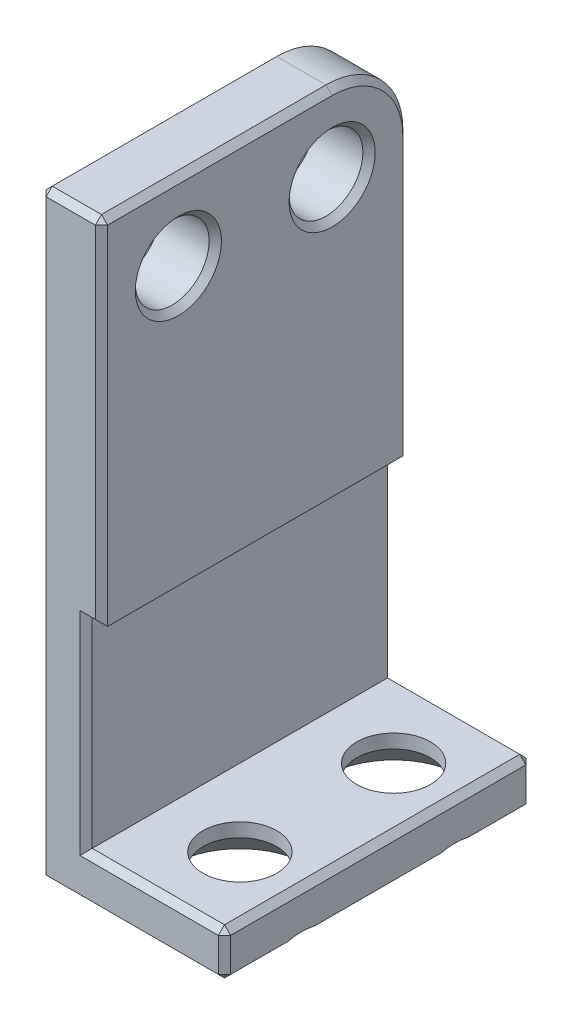
SolidWorks part; units mm, degrees
material "7075-T6"
ref_plane "Front Plane" through (0, 0, 0) normal (0, 0, 1) x (1, 0, 0)
ref_plane "Top Plane" through (0, 0, 0) normal (0, 1, 0) x (1, 0, 0)
ref_plane "Right Plane" through (0, 0, 0) normal (1, 0, 0) x (0, 0, -1)
sketch "Sketch1" plane through (0, 0, 0) normal (0, 1, 0) x (1, 0, 0)
  line L1 (0, 0) -> (2, 0)
  line L2 (0, 0) -> (0, 10)
  line L3 (0, 10) -> (2, 10)
  line L4 (2, 0) -> (2, 10)
  dimension "D1" = 10
  dimension "D2" = 2
extrude "Boss-Extrude1" add sketch "Sketch1" along normal blind 19.5
sketch "Sketch2" plane through (2, 0, 0) normal (1, 0, 0) x (0, 0, -1)
  line L0 (7.5, 17) -> (2.5, 17) construction
  line L1 (0, 0) -> (10, 0) construction
  line L2 (0, 19.5) -> (10, 19.5) construction
  circle A0 centre (2.5, 17) radius 1.2
  circle A1 centre (7.5, 17) radius 1.2
  point P4 (5, 17)
  point P7 (5, 0)
  dimension "D2" = 2.4
  dimension "D1" = 2.5
  dimension "D3" = 5
extrude "Cut-Extrude1" cut sketch "Sketch2" against normal blind 20
sketch "Sketch3" plane through (2, 0, 0) normal (1, 0, 0) x (0, 0, -1)
  line L0 (10, 19.5) -> (10, 0) construction
  line L1 (0, 0) -> (10, 0)
  line L2 (0, 0) -> (0, 1.5)
  line L3 (0, 1.5) -> (10, 1.5)
  line L4 (10, 0) -> (10, 1.5)
  dimension "D1" = 1.5
extrude "Boss-Extrude2" add sketch "Sketch3" along normal blind 4
sketch "Sketch4" plane through (2, 0, 0) normal (1, 0, 0) x (0, 0, -1)
  line L0 (10, 19.5) -> (10, 1.5) construction
  line L1 (0, 1.5) -> (10, 1.5)
  line L2 (0, 1.5) -> (0, 8)
  line L3 (0, 8) -> (10, 8)
  line L4 (10, 1.5) -> (10, 8)
  dimension "D1" = 6.5
extrude "Cut-Extrude2" cut sketch "Sketch4" against normal blind 0.5
hole_wizard "Hole size slotted countersunk wood screw type 0" positions "Sketch5" profile "Sketch6" countersink size "M2" standard "GB" end condition up to next
sketch "Sketch5" plane through (0, 0, 0) normal (0, -1, 0) x (-1, 0, 0)
  line L0 (-4, 2.5) -> (-4, 7.5)
  line L2 (-6, 0) -> (-6, 10) construction
  line L3 (-6, 10) -> (0, 10) construction
  point P0 (-4, 2.5)
  point P2 (-4, 7.5)
  dimension "D1" = 2
  dimension "D2" = 5
  dimension "D3" = 2.5
sketch "Sketch6" plane through (4, 0, -2.5) normal (1, 0, 0) x (0, 0, -1)
  line L0 (0, 0) -> (0, 1.5)
  line L1 (0, 1.5) -> (1.2, 1.5)
  line L2 (1.2, 1.5) -> (1.2, 1.05)
  line L3 (1.2, 1.05) -> (2.25, 0)
  line L5 (2.25, 0) -> (0, 0)
  line L6 (-1.2, 1.05) -> (-2.25, 0) construction
  line L11 (0, -6.35) -> (0, 107.95) construction
  dimension "通孔孔直径" = 2.4
  dimension "通孔孔深度" = 1.5
  dimension "近端锥形沉头孔直径" = 4.5
  dimension "近端锥形沉头孔角度" = 90
fillet "Fillet1" radius 2.5 1 edges at (1, 19.5, -10)
chamfer "Chamfer1" distance 0.2 angle 45 28 edges at (0, 17, -8.7) (0, 17, -3.7) (6, 0, -5) (2, 19.5, -3.75) (2, 18.7678, -9.2678) (3, 0, -10) (6, 0, -9.2654) (6, 0.75, -10) (2, 12.5, -10) (1.75, 8, -10) (1.5, 4.75, -10) (3.75, 1.5, -10) (3.75, 1.5, 0) (1.5, 4.75, 0) (1.75, 8, 0) (2, 13.75, 0) (1, 19.5, 0) (0, 9.75, 0) (0, 19.5, -3.75) (0, 18.7678, -9.2678) (0, 8.5, -10) (0, 0, -5) (3, 0, 0) (6, 0, -0.7346) (6, 0.75, 0) (6, 1.5, -5) (2, 17, -3.7) (2, 17, -8.7)
